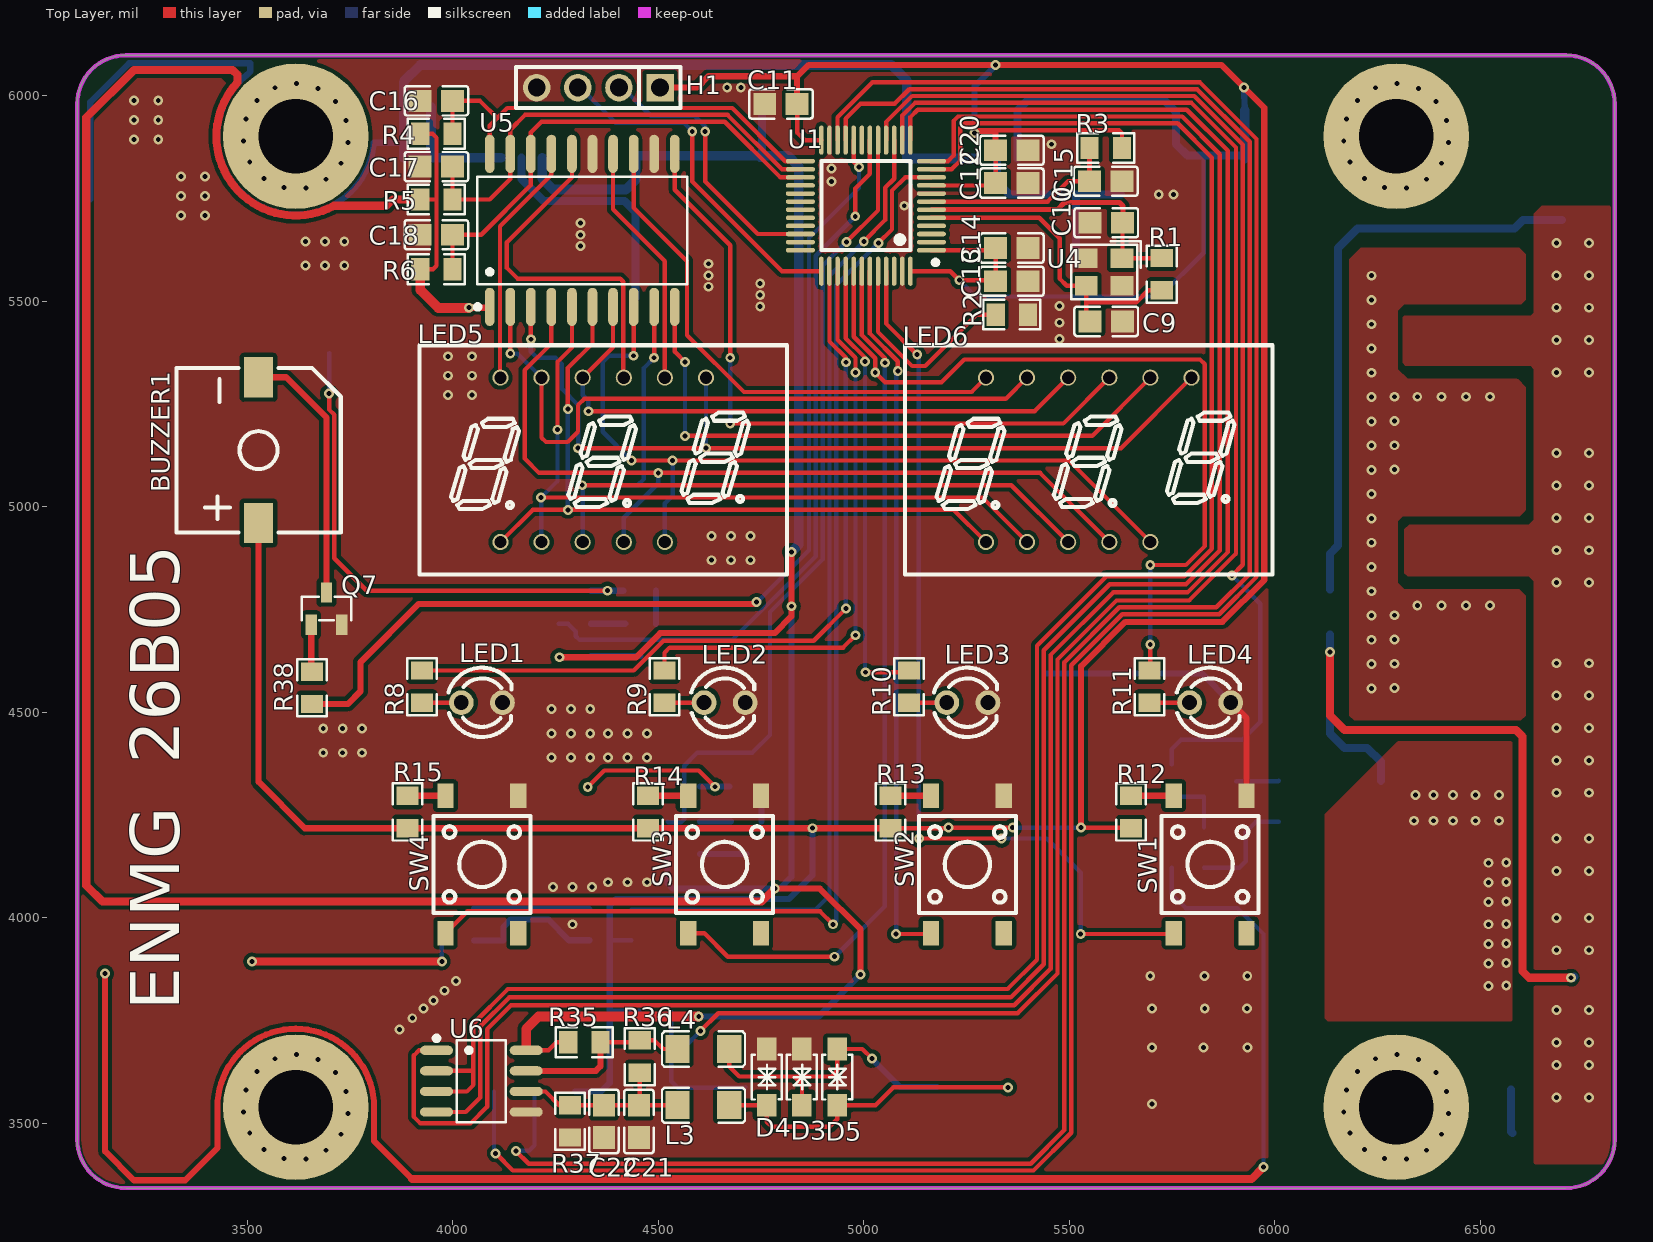
[diagram p0: Top Layer view]
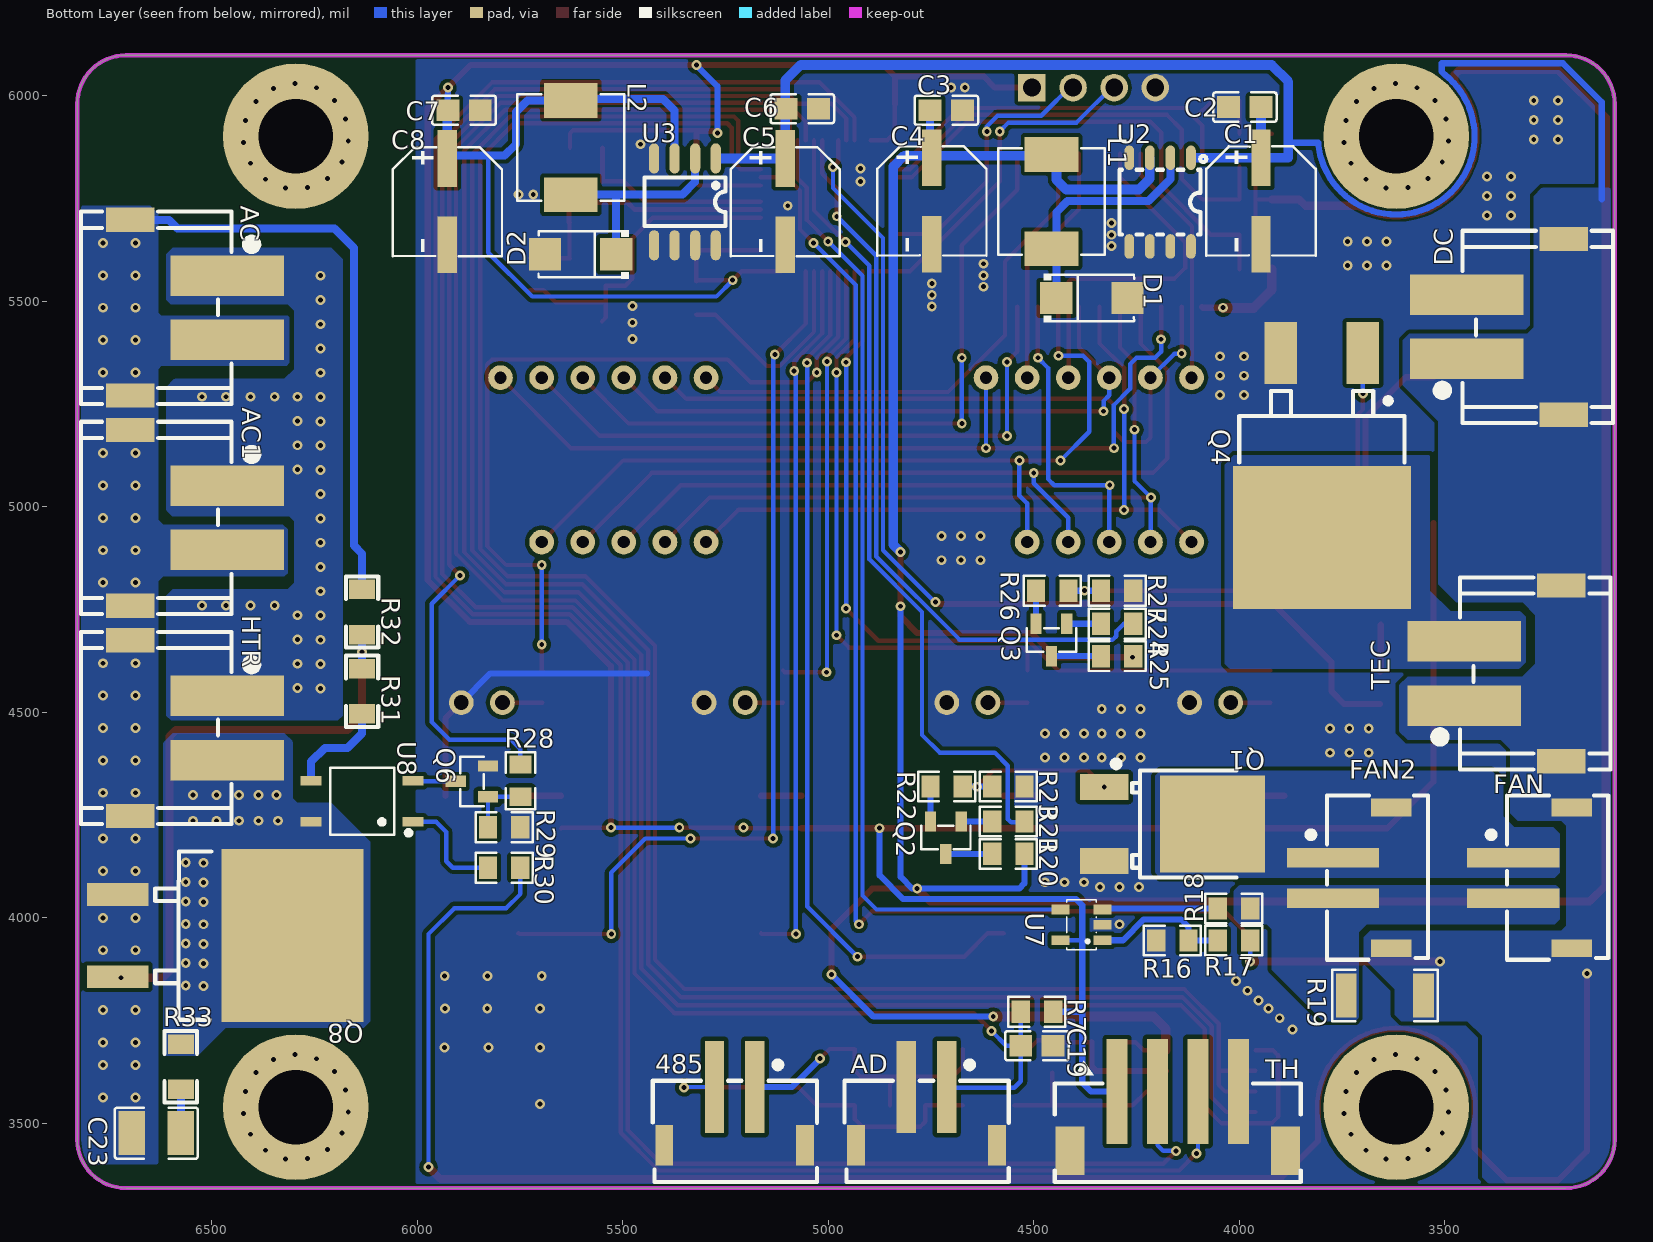
[diagram p1: Bottom Layer view, seen from below]
# Altium PCB MISC82750.pcbdoc (part 1 of 3)
Units mil, origin at the board's own origin, x right, y up, seen from the top; angles counter-clockwise.
Board outline 3740.2 x 2755.9 mil, 2 copper layers (Top Layer, Bottom Layer), stack 62.2 mil thick; 106 components, 84 nets, 362 pads, 334 vias.

## Layer stack, top to bottom
Top Solder Mask Layer: solder mask 0.4, Dk 3.3
Top Layer: signal copper 1.4
Dielectric1: surface 59.4, FR4, Dk 4.5
Bottom Layer: signal copper 1.4
Bottom Solder Mask Layer: solder mask 0.4, Dk 3.3

## Board outline
3204.7,6098.4 ccw(c3204.7,5980.3) 3086.6,5980.3 3086.6,3460.6 ccw(c3204.7,3460.6) 3204.7,3342.5 6708.7,3342.5 ccw(c6708.7,3460.6) 6826.8,3460.6 6826.8,5980.3 ccw(c6708.7,5980.3) 6708.7,6098.4

## Design rules (kind name [scope] priority, off if disabled: settings)
BoardOutlineClearance copperThickness1oz [All] p0: genericclearance=10 ignorepadtopadclearanceinfootprint=FALSE except(0: Arc-SplitContinuation Track-SplitContinuation SMDPad-SplitContinuation THPad-SplitContinuation Via-SplitContinuation Fill-SplitContinuation Poly-SplitContinuation Region-SplitContinuation Text-SplitContinuation)
BoardOutlineClearance copperThickness2oz [All] p0: genericclearance=10 ignorepadtopadclearanceinfootprint=FALSE except(0: Arc-SplitContinuation Track-SplitContinuation SMDPad-SplitContinuation THPad-SplitContinuation Via-SplitContinuation Fill-SplitContinuation Poly-SplitContinuation Region-SplitContinuation Text-SplitContinuation)
BoardOutlineClearance Plane_innerPlane [All] p0: genericclearance=10 ignorepadtopadclearanceinfootprint=FALSE except(0: Arc-SplitContinuation Track-SplitContinuation SMDPad-SplitContinuation THPad-SplitContinuation Via-SplitContinuation Fill-SplitContinuation Poly-SplitContinuation Region-SplitContinuation Text-SplitContinuation)
BoardOutlineClearance Copper_copperRegion [All] p0: genericclearance=10 ignorepadtopadclearanceinfootprint=FALSE except(0: Arc-SplitContinuation Track-SplitContinuation SMDPad-SplitContinuation THPad-SplitContinuation Via-SplitContinuation Fill-SplitContinuation Poly-SplitContinuation Region-SplitContinuation Text-SplitContinuation)
BoardOutlineClearance otherClearance [All] p0: genericclearance=10 ignorepadtopadclearanceinfootprint=FALSE except(0: Arc-SplitContinuation Track-SplitContinuation SMDPad-SplitContinuation THPad-SplitContinuation Via-SplitContinuation Fill-SplitContinuation Poly-SplitContinuation Region-SplitContinuation Text-SplitContinuation)
Clearance copperThickness1oz [All] p1: gap=7 ignorepadtopadclearanceinfootprint=FALSE
Clearance copperThickness2oz [All] p1: gap=7 ignorepadtopadclearanceinfootprint=FALSE
Clearance Plane_innerPlane [All] p1: gap=7 ignorepadtopadclearanceinfootprint=FALSE
Clearance Copper_copperRegion [All] p1: gap=7 ignorepadtopadclearanceinfootprint=FALSE
Clearance otherClearance [All] p1: gap=7 ignorepadtopadclearanceinfootprint=FALSE
DiffPairsRouting differentialPair [All] p1: maxuncoupledlength=10 minlimit=6 maxlimit=Infinity mostfreqgap=6 toplayer_minwidth=5 toplayer_prefwidth=10 toplayer_maxwidth=100 bottomlayer_minwidth=5 bottomlayer_prefwidth=10 bottomlayer_maxwidth=100
PasteMaskExpansion pasteMaskExpansion [All] p1: expansion=0
PlaneConnect innerPlane [All] p1: planeconnectstyle=Relief reliefexpansion=20 reliefentries=4 reliefconductorwidth=10 reliefairgap=10
PolygonConnect copperRegion [All] p1: connectstyle=Direct reliefentries=4 reliefconductorwidth=10 polygonreliefangle="90 Angle" airgapwidth=10
RoutingVias viaSize [All] p1: viastyle="Through Hole" holewidth=12.0078 minholewidth=11.811 maxholewidth=248.0314 width=12.0078 minwidth=11.811 maxwidth=248.0314
SolderMaskExpansion solderMaskExpansion [IsVia] p1: useseparateexpansions=TRUE expansion=-1000 expansionbottom=-1000
SolderMaskExpansion solderMaskExpansion [All] p2: useseparateexpansions=TRUE expansion=2 expansionbottom=2
Width copperThickness1oz [All] p1: maxlimit=100 minlimit=5 preferedwidth=10
Width copperThickness2oz [All] p1: maxlimit=100 minlimit=8 preferedwidth=10
Width trackWidth1 [All] p1: maxlimit=100 minlimit=5 preferedwidth=30

## Components (designator, comment, footprint, x,y, rotation, side; value= is the part's Value field where it differs from the comment)
485 "XH2.54-2P立贴" CONN-SMD_2P_A2501WV-S#1 5227.5,3517.5 r180 bottom
AC "VH3.96-2P 立贴" CONN-SMD_2P-P3.96_HCTL_HC-VH-2ALT#1 6580,5484.3 r270 bottom
AC1 "VH3.96-2P 立贴" CONN-SMD_2P-P3.96_HCTL_HC-VH-2ALT#2 6580,4973 r270 bottom
AD "XH2.54-2P立贴" CONN-SMD_2P_A2501WV-S#2 4760.9,3517.5 r180 bottom
BUZZER1 "2.7kHz" BUZ-SMD_L9.6-W9.6-LS10.0-R 3527.6,5137.8 r270 top
C1 "220uF" CAP-SMD_BD6.3-L6.6-W6.6-FD#1 3947.2,5744 r270 bottom
C2 "100nF" C0805#1 3986.5,5972.4 r0 bottom
C3 "100nF" C0805#2 4712.6,5964.6 r0 bottom
C4 "220uF" CAP-SMD_BD6.3-L6.6-W6.6-FD#1 4747.8,5744 r270 bottom
C5 "220uF" CAP-SMD_BD6.3-L6.6-W6.6-FD#2 5104.6,5742.2 r270 bottom
C6 "100nF" C0805#2 5063,5968.5 r180 bottom
C7 "100nF" C0805#1 5885.8,5964.6 r0 bottom
C8 "220uF" CAP-SMD_BD6.3-L6.6-W6.6-FD#2 5926.6,5742.2 r270 bottom
C9 "20pF" C0805#2 5589.8,5451 r180 top
C10 "20pF" C0805#2 5589.8,5691 r0 top
C11 "100nF" C0805#1 4798.3,5980 r0 top
C12 "100nF" C0805#3 5360,5787.5 r180 top
C13 "100nF" C0805#3 5360,5548.7 r180 top
C14 "100nF" C0805#3 5360,5629.4 r180 top
C15 "100nF" C0805#2 5588.6,5791.9 r180 top
C16 "100pF" C0805#1 3960,5987.5 r0 top
C17 "100pF" C0805#1 3960,5827.5 r0 top
C18 "100pF" C0805#1 3960,5662 r0 top
C19 "100nF" C0805#1 4492.1,3689 r0 bottom
C20 "100nF" C0805#3 5360,5867.5 r180 top
C21 "100nF" C0805#1 4452.9,3504.8 r90 top
C22 "100nF" C0805#1 4367.9,3504.8 r90 top
C23 "10nF" C1210 6634.5,3476.4 r180 bottom
D1 "SS34" SMA_L4.3-W2.6-LS5.2-RD 4358.3,5507.9 r180 bottom
D2 "SS34" SMA_L4.3-W2.6-LS5.2-RD 5602.4,5614.2 r0 bottom
D3 "SMF36CA" SOD-123_L2.7-W1.8-LS3.7-BI 4849.5,3612.5 r90 top
D4 "SMF36CA" SOD-123_L2.7-W1.8-LS3.7-BI 4763.9,3612.5 r90 top
D5 "SMF36CA" SOD-123_L2.7-W1.8-LS3.7-BI 4935,3612.5 r90 top
DC "VH3.96-2P 立贴" CONN-SMD_2P-P3.96_HCTL_HC-VH-2ALT#3 3328.7,5437.5 r90 bottom
FAN "XH2.54-2P立贴" CONN-SMD_2P_A2501WV-S#3 3262.4,4097.2 r90 bottom
FAN2 "XH2.54-2P立贴" CONN-SMD_2P_A2501WV-S#4 3700.8,4097.2 r90 bottom
H1 "PZ254V-11-04P" HDR-TH_4P-P2.54-V-M 4354.3,6019.7 r180 top
HTR "VH3.96-2P 立贴" CONN-SMD_2P-P3.96_HCTL_HC-VH-2ALT#2 6580,4461.8 r270 bottom
L1 "68uH" IND-SMD_L7.1-W6.6_H5.0 4456.7,5742.6 r270 bottom
L2 "68uH" IND-SMD_L7.1-W6.6_H5.0 5626,5874 r270 bottom
L3 "22uH" L1206 4610,3544.2 r0 top
L4 "22uH" L1206 4610,3680.8 r0 top
LED1 "3mmFIR" LED-TH_BD3.0-P2.54-FD 4070.9,4523.6 r0 top
LED2 "3mmFIR" LED-TH_BD3.0-P2.54-FD 4661.4,4523.6 r0 top
LED3 "3mmFIR" LED-TH_BD3.0-P2.54-FD 5252,4523.6 r0 top
LED4 "3mmFIR" LED-TH_BD3.0-P2.54-FD 5842.5,4523.6 r0 top
LED5 "SP420361N" LED-SEG-TH_SP420361N 4366.1,5114.2 r270 top
LED6 "SP420361N" LED-SEG-TH_SP420361N 5547.2,5114.2 r270 top
Q1 "NCE0140K2-VB" TO-252-3_L6.6-W6.1-P4.58-LS10.1-BR 4196.9,4228.3 r0 bottom
Q2 "SS8050(RANGE:200-350)" SOT-23-3_L2.9-W1.3-P1.90-LS2.4-BR#1 4713.9,4195 r90 bottom
Q3 "SS8050(RANGE:200-350)" SOT-23-3_L2.9-W1.3-P1.90-LS2.4-BR#2 4456.9,4675.9 r90 bottom
Q4 "HYG025N06LS1B" TO-263-2_L10.2-W8.7-P5.08-LS15.1-BR 3799.2,5149.6 r90 bottom
Q6 "SS8050(RANGE:200-350)" SOT-23-3_L2.9-W1.3-P1.90-LS2.4-BR#2 5867,4331.9 r180 bottom
Q7 "SS8050(RANGE:200-350)" SOT-23-3_L2.9-W1.3-P1.90-LS2.4-BR#1 3693,4752.4 r270 top
Q8 "BTA216B-600D-JSM" TO-263-3_L10.2-W9.2-P5.08-LS15.4-BR 6515.7,3956.7 r0 bottom
R1 "1MΩ" R0805#1 5724.8,5566 r270 top
R2 "10kΩ" R0805#1 5360,5467.5 r180 top
R3 "10kΩ" R0805#2 5588.6,5873.1 r0 top
R4 "10kΩ" R0805#1 3960,5907.5 r180 top
R5 "10kΩ" R0805#1 3960,5747.5 r180 top
R6 "10kΩ" R0805#1 3960,5578.1 r180 top
R7 "10kΩ" R0805#1 4492.1,3771.7 r180 bottom
R8 "100Ω" R0805#2 3925,4562.5 r90 top
R9 "100Ω" R0805#2 4515,4562.5 r90 top
R10 "100Ω" R0805#2 5110,4562.5 r90 top
R11 "100Ω" R0805#2 5695,4562.5 r90 top
R12 "4.7kΩ" R0805#2 5650,4257.5 r270 top
R13 "4.7kΩ" R0805#2 5065,4257.5 r270 top
R14 "4.7kΩ" R0805#2 4475,4257.5 r270 top
R15 "4.7kΩ" R0805#2 3890,4257.5 r270 top
R16 "24kΩ" R0805#1 4163,3944.9 r0 bottom
R17 "1kΩ" R0805#3 4013,3944.9 r180 bottom
R18 "1kΩ" R0805#3 4013,4022.7 r180 bottom
R19 "10mΩ" R2010 3645.7,3811 r180 bottom
R20 "4.7kΩ" R0805#3 4561.9,4155.6 r0 bottom
R21 "1kΩ" R0805#3 4561.9,4234.4 r0 bottom
R22 "10K" R0805#1 4711.9,4319.4 r180 bottom
R23 "10kΩ" R0805#3 4561.9,4319.4 r0 bottom
R24 "1kΩ" R0805#3 4296.9,4715.3 r0 bottom
R25 "4.7kΩ" R0805#3 4296.9,4636.6 r0 bottom
R26 "10K" R0805#3 4455,4795.9 r180 bottom
R27 "10kΩ" R0805#3 4296.9,4795.9 r0 bottom
R28 "10K" R0805#1 5748.8,4333.8 r270 bottom
R29 "10K" R0805#2 5788.2,4220.5 r180 bottom
R30 "10K" R0805#2 5788.2,4122 r180 bottom
R31 "51Ω" R0204 6133.9,4551.2 r90 bottom
R32 "150Ω" R0204 6133.9,4744.1 r90 bottom
R33 "120Ω" R0204 6574.8,3637.8 r90 bottom
R35 "47kΩ" R0805#1 4320,3697.5 r180 top
R36 "12kΩ" R0805#2 4455,3662.5 r90 top
R37 "47kΩ" R0805#3 4285,3504.8 r90 top
R38 "1kΩ" R0805#1 3657.5,4559.5 r90 top
SW1 "1TS005F-2500-5001" SW-SMD_4P-L6.0-W6.0-P4.50-LS9.0-H2.5#1 5842.5,4129.9 r90 top
SW2 "1TS005F-2500-5001" SW-SMD_4P-L6.0-W6.0-P4.50-LS9.0-H2.5#2 5252,4129.9 r90 top
SW3 "1TS005F-2500-5001" SW-SMD_4P-L6.0-W6.0-P4.50-LS9.0-H2.5#1 4661.4,4129.9 r90 top
SW4 "1TS005F-2500-5001" SW-SMD_4P-L6.0-W6.0-P4.50-LS9.0-H2.5#2 4070.9,4129.9 r90 top
TEC "VH3.96-2P 立贴" CONN-SMD_2P-P3.96_HCTL_HC-VH-2ALT#4 3334.6,4594.5 r90 bottom
TH "HX 2.54-4P LT" CONN-SMD_4P-P2.50_HX-2.54-4P-LT 4149.6,3505.7 r180 bottom
U1 "GD32F103C8T6" TQFP-48_L7.0-W7.0-P0.50-LS9.0-BL 5005,5732.5 r90 top
U2 "XL1509-5.0" SOIC-8_L4.9-W3.9-P1.27-LS6.0-TR 4192.6,5741.2 r180 bottom
U3 "XL1509-3.3E1" SOP-8_L4.9-W3.9-P1.27-LS6.0-BL 5348.6,5741.8 r0 bottom
U4 "8MHz" CRYSTAL-SMD_4P-L3.2-W2.5-BL 5584.8,5571 r180 top
U5 "TM1620" SOIC-20_L13.0-W7.6-P1.27-LS10.3-BL 4315,5672.5 r0 top
U6 "MAX485ESA(UMW)" SOP-8_L5.0-W4.0-P1.27-LS6.0-BL 4069.6,3602.7 r270 top
U7 "LMV321" SOT-23-5_L3.0-W1.7-P0.95-LS2.8-BR 4383.7,3983 r180 bottom
U8 "ELM3083(TA)-V" SOP-4_L4.4-W4.0-P2.54-LS7.0-TL 6133.9,4283.5 r0 bottom

## Footprints (in the part's own frame and the unit in brackets; to place one, negate y for a bottom-side part, rotate by r counter-clockwise, add the part's x,y. Pads: shape width x height; smd on the part's side, far side on the other; paste and mask are expansions set on the pad)
BUZ-SMD_L9.6-W9.6-LS10.0-R [mil]
  rect 98.4x70.9 smd: 1(177.2,0) 2(-177.2,0)
  silkscreen extent -200,-200 200,200
C0805#1 [mil]
  rect 55.5x53.1 smd paste-3937 mask+2: 1(-39.3,0) 2(39.4,0)
  silkscreen extent -77,-36 77,36
C0805#2 [mil]
  rect 55.5x53.1 smd paste-3937 mask+2: 1(-39.4,0) 2(39.4,0)
  silkscreen extent -77,-36 77,36
C0805#3 [mil]
  rect 55.5x53.1 smd paste-3937 mask+2: 1(-39.4,0) 2(39.3,0)
  silkscreen extent -77,-36 77,36
C1210 [mil]
  rect 64.4x106.3 smd paste-3937 mask+2: 1(-59.8,0) 2(59.7,0)
  silkscreen extent -101,-62 101,62
CAP-SMD_BD6.3-L6.6-W6.6-FD#1 [mil]
  rect 137.8x47.2 smd: 1(-105.1,0) 2(105.1,0)
  silkscreen extent -133,-133 133,133
CAP-SMD_BD6.3-L6.6-W6.6-FD#2 [mil]
  rect 137.8x47.2 smd: 1(-105.2,0) 2(105.1,0)
  silkscreen extent -133,-133 133,133
CONN-SMD_2P-P3.96_HCTL_HC-VH-2ALT#1 [mil]
  rect 98.4x275.6 smd paste+0 mask+2: 1(-77.9,118.1) 2(78,118.1)
  rect 59.1x118.1 smd paste+0 mask+2: 3(213.8,-118.1) 4(-213.7,-118.1)
  silkscreen extent -234,-238 234,189
CONN-SMD_2P-P3.96_HCTL_HC-VH-2ALT#2 [mil]
  rect 98.4x275.6 smd paste+0 mask+2: 1(-78,118.1) 2(77.9,118.1)
  rect 59.1x118.1 smd paste+0 mask+2: 3(213.8,-118.1) 4(-213.8,-118.1)
  silkscreen extent -234,-238 234,189
CONN-SMD_2P-P3.96_HCTL_HC-VH-2ALT#3 [mil]
  rect 98.4x275.6 smd paste+0 mask+2: 1(-77.9,118.2) 2(78,118.2)
  rect 59.1x118.1 smd paste+0 mask+2: 3(213.8,-118.1) 4(-213.8,-118.1)
  silkscreen extent -234,-238 234,189
CONN-SMD_2P-P3.96_HCTL_HC-VH-2ALT#4 [mil]
  rect 98.4x275.6 smd paste+0 mask+2: 1(-78,118.2) 2(77.9,118.2)
  rect 59.1x118.1 smd paste+0 mask+2: 3(213.8,-118.1) 4(-213.8,-118.1)
  silkscreen extent -234,-238 234,189
CONN-SMD_2P_A2501WV-S#1 [mil]
  rect 47.2x224.4 smd paste+0 mask+2: 1(49.2,70.9) 2(-49.2,70.9)
  rect 43.3x98.4 smd paste+0 mask+2: 3(-171.3,-70.8) 4(171.2,-70.8)
  silkscreen extent -199,-160 200,133
CONN-SMD_2P_A2501WV-S#2 [mil]
  rect 47.2x224.4 smd paste+0 mask+2: 1(49.2,70.9) 2(-49.3,70.9)
  rect 43.3x98.4 smd paste+0 mask+2: 3(-171.3,-70.8) 4(171.2,-70.8)
  silkscreen extent -199,-160 200,133
CONN-SMD_2P_A2501WV-S#3 [mil]
  rect 47.2x224.4 smd paste+0 mask+2: 1(49.2,70.8) 2(-49.3,70.8)
  rect 43.3x98.4 smd paste+0 mask+2: 3(-171.3,-70.9) 4(171.2,-70.9)
  silkscreen extent -199,-160 200,133
CONN-SMD_2P_A2501WV-S#4 [mil]
  rect 47.2x224.4 smd paste+0 mask+2: 1(49.2,70.9) 2(-49.3,70.9)
  rect 43.3x98.4 smd paste+0 mask+2: 3(-171.3,-70.9) 4(171.2,-70.9)
  silkscreen extent -199,-160 200,133
CONN-SMD_4P-P2.50_HX-2.54-4P-LT [mil]
  rect 51.2x255.9 smd paste+0 mask+2: 1(-147.6,71.9) 2(-49.2,71.9) 3(49.2,71.9) 4(147.6,71.9)
  rect 70.9x118.1 smd paste+0 mask+2: 5(261.8,-71.8) 6(-261.8,-71.8)
  silkscreen extent -299,-149 299,147
CRYSTAL-SMD_4P-L3.2-W2.5-BL [mil]
  rect 55.1x47.2 smd: 1(-43.3,-33.5) 2(43.3,-33.5) 3(43.3,33.4) 4(-43.3,33.4)
  silkscreen extent -89,-75 80,66
HDR-TH_4P-P2.54-V-M [mil]
  rect 66.9x66.9 hole 43.3: 1(-150,0)
  round 66.9 hole 43.3: 2(-50,0) 3(50,0) 4(150,0)
  silkscreen extent -200,-50 200,50
IND-SMD_L7.1-W6.6_H5.0 [mil]
  rect 84.6x130.7 smd: 1(-114.7,0) 2(114.7,0)
  silkscreen extent -130,-130 130,130
L1206 [mil]
  rect 58.5x68 smd paste-3937 mask+2: 1(-62.7,0) 2(62.7,0)
  silkscreen extent -101,-43 101,43
LED-SEG-TH_SP420361N [mil]
  round 39.4 / inner round 39.4 / far side round 60 hole 30: 1(200,-250) 2(200,-150) 3(200,-50) 4(200,50) 5(200,150) 7(-200,250) 8(-200,150) 9(-200,50) 10(-200,-50) 11(-200,-150) 12(-200,-250)
  silkscreen extent -279,-447 279,447
LED-TH_BD3.0-P2.54-FD [mil]
  round 60 hole 36: 1(-50,0) 2(50,0)
  silkscreen extent -81,-84 72,85
R0204 [mil]
  rect 47.2x63 smd paste+0 mask+2: 1(-55.1,0) 2(55.1,0)
  silkscreen extent -87,-39 87,39
R0805#1 [mil]
  rect 44.6x54.2 smd paste-3937 mask+2: 1(-39.4,0) 2(39.3,0)
  silkscreen extent -69,-36 69,36
R0805#2 [mil]
  rect 44.6x54.2 smd paste-3937 mask+2: 1(-39.4,0) 2(39.4,0)
  silkscreen extent -69,-36 69,36
R0805#3 [mil]
  rect 44.6x54.2 smd paste-3937 mask+2: 1(-39.3,0) 2(39.4,0)
  silkscreen extent -69,-36 69,36
R2010 [mil]
  rect 50.5x106.3 smd paste-3937 mask+2: 1(-94.1,0) 2(94.2,0)
  silkscreen extent -128,-62 128,62
SMA_L4.3-W2.6-LS5.2-RD [mil]
  rect 78.7x78.7 smd: 1(-86.6,0) 2(86.6,0)
  silkscreen extent -117,-59 102,59
SOD-123_L2.7-W1.8-LS3.7-BI [mil]
  rect 55.1x47.2 smd: 1(-68.3,0) 2(68.3,0)
  silkscreen extent -54,-36 54,36
SOIC-8_L4.9-W3.9-P1.27-LS6.0-TR [mil]
  oval 23.6x59.8 smd: 1(75,107.9) 2(25,107.9) 3(-25,107.9) 4(-75,107.9) 5(-75,-107.8) 6(-25,-107.8) 7(25,-107.8) 8(75,-107.8)
  silkscreen extent -98,-79 113,112
SOIC-20_L13.0-W7.6-P1.27-LS10.3-BL [mil]
  oval 23.4x92.9 smd: 1(-225,-186.2) 2(-175,-186.2) 3(-125,-186.2) 4(-75,-186.2) 5(-25,-186.2) 6(25,-186.2) 7(75,-186.2) 8(125,-186.2) 9(175,-186.2) 10(225,-186.2) 11(225,186.2) 12(175,186.2) 13(125,186.2) 14(75,186.2) 15(25,186.2) 16(-25,186.2) 17(-75,186.2) 18(-125,186.2) 19(-175,186.2) 20(-225,186.2)
  silkscreen extent -260,-192 255,131
SOP-4_L4.4-W4.0-P2.54-LS7.0-TL [mil]
  rect 51.2x23.4 smd: 1(-124.1,50) 2(-124.1,-50) 3(124,-50) 4(124,50)
  silkscreen extent -119,-82 78,82
SOP-8_L4.9-W3.9-P1.27-LS6.0-BL [mil]
  oval 24.8x73.4 smd: 1(-75,-105.6) 2(-25,-105.6) 3(25,-105.6) 4(75,-105.6) 5(75,105.7) 6(25,105.7) 7(-25,105.7) 8(-75,105.7)
  silkscreen extent -98,-59 98,58
SOP-8_L5.0-W4.0-P1.27-LS6.0-BL [mil]
  oval 22.6x80.1 smd: 1(-75,-109) 2(-25,-109) 3(25,-109) 4(75,-109) 5(75,109) 6(25,109) 7(-25,109) 8(-75,109)
  silkscreen extent -110,-115 100,60
SOT-23-3_L2.9-W1.3-P1.90-LS2.4-BR#1 [mil]
  rect 49.2x27.6 smd: 1(39.4,-37.4) 2(39.4,37.4) 3(-39.4,0)
  silkscreen extent -29,-60 29,60
SOT-23-3_L2.9-W1.3-P1.90-LS2.4-BR#2 [mil]
  rect 49.2x27.6 smd: 1(39.4,-37.4) 2(39.4,37.4) 3(-39.3,0)
  silkscreen extent -29,-60 29,60
SOT-23-5_L3.0-W1.7-P0.95-LS2.8-BR [mil]
  rect 43.3x23.6 smd: 1(51.1,-37.4) 2(51.1,0) 3(51.1,37.4) 4(-51.2,37.4) 5(-51.2,-37.4)
  silkscreen extent -36,-61 35,61
SW-SMD_4P-L6.0-W6.0-P4.50-LS9.0-H2.5#1 [mil]
  rect 59.1x39.4 smd: 1(-167.3,88.6) 2(167.3,88.6) 3(-167.3,-88.6) 4(167.3,-88.6)
  silkscreen extent -118,-118 118,118
SW-SMD_4P-L6.0-W6.0-P4.50-LS9.0-H2.5#2 [mil]
  rect 59.1x39.4 smd: 1(-167.3,88.6) 2(167.3,88.6) 3(-167.3,-88.5) 4(167.3,-88.5)
  silkscreen extent -118,-118 118,118
TO-252-3_L6.6-W6.1-P4.58-LS10.1-BR [mil]
  rect 118.1x63 smd: 1(131.5,-90) 2(131.5,89.9)
  rect 255.9x236.2 smd: 3(-131.6,0)
  silkscreen extent -190,-154 110,130
TO-263-2_L10.2-W8.7-P5.08-LS15.1-BR [mil]
  rect 150x78.7 smd: 1(224.5,-100) 3(224.6,100)
  rect 348x433.1 smd: 4(-224.5,0)
  silkscreen extent -41,-201 132,201
TO-263-3_L10.2-W9.2-P5.08-LS15.4-BR [mil]
  rect 149.6x55.1 smd: 1(212.6,-100) 3(212.6,100)
  rect 346.5x421.3 smd: 2(-212.5,0)
  silkscreen extent -15,-205 121,205
TQFP-48_L7.0-W7.0-P0.50-LS9.0-BL [mil]
  oval 11x70.9 smd: 1(-108.3,-159.5) 2(-88.6,-159.5) 3(-68.9,-159.5) 4(-49.2,-159.5) 5(-29.5,-159.5) 6(-9.8,-159.5) 7(9.9,-159.5) 8(29.5,-159.5) 9(49.2,-159.5) 10(68.9,-159.5) 11(88.6,-159.5) 12(108.3,-159.5) 25(108.3,159.4) 26(88.6,159.4) 27(68.9,159.4) 28(49.2,159.4) 29(29.5,159.4) 30(9.9,159.4) 31(-9.8,159.4) 32(-29.5,159.4) 33(-49.2,159.4) 34(-68.9,159.4) 35(-88.6,159.4) 36(-108.3,159.4)
  oval 70.9x11 smd: 13(159.5,-108.3) 14(159.5,-88.6) 15(159.5,-68.9) 16(159.5,-49.2) 17(159.5,-29.6) 18(159.5,-9.9) 19(159.5,9.8) 20(159.5,29.5) 21(159.5,49.2) 22(159.5,68.9) 23(159.5,88.5) 24(159.5,108.2) 37(-159.4,108.2) 38(-159.4,88.5) 39(-159.4,68.9) 40(-159.4,49.2) 41(-159.4,29.5) 42(-159.4,9.8) 43(-159.4,-9.9) 44(-159.4,-29.6) 45(-159.4,-49.2) 46(-159.4,-68.9) 47(-159.4,-88.6) 48(-159.4,-108.3)
  silkscreen extent -144,-175 108,108

## Free pads (board coordinates)
  round 354.3 / inner round 196.9 / far side round 354.3 hole 181.1: 1(3618.1,5901.6) 2(6295.3,5901.6) 3(6295.3,3539.4) 4(3618.1,3539.4)

## Via types
v1: diameter 24, hole 12, Top Layer to Bottom Layer, 334 vias

## Nets (pads, with @x,y where several pads share a name; then routed paths per layer and width w, separated by ;. In a path a pad name is that pad's centre, name@x,y a point inside that pad or via, vN(x,y) a via of type N, cw(c..) or ccw(c..) an arc to the next point about the centre after c; other vN are vias at no path point)
1: LED5.12 U5.17 | length 596.7
  Top Layer w10.6: LED5.12@4116.1,5314.2 4115,5315.3 4115,5682.5 4240,5807.5 U5.17@4240,5858.7
2: LED5.9 U5.16 | length 874.3
  Top Layer w10.6: U5.16@4290,5858.7 4290,5801.9 4131.7,5643.5 4131.7,5580.9 4157.5,5555.1 4407.5,5555.1 4415,5547.6 4415,5315.3 LED5.9@4416.1,5314.2
3: LED5.8 U5.14 | length 596.7
  Top Layer w10.6: U5.14@4390,5858.7 4390,5723.6 4516.1,5597.5 LED5.8@4516.1,5314.2
4: LED6.12 U5.13 | length 1294.1
  Top Layer w10.6: U5.13@4440,5858.7 4440,5727.5 4570,5597.5 4570,5417.5 4708.4,5279.1 5262.2,5279.1 LED6.12@5297.2,5314.2
5: LED6.9 U5.11 | length 1680.6
  Top Layer w10.6: U5.11@4540,5858.7 4540,5771 4675,5636 v1(4675,5362.5) ; v1(4675,5202.5) 5485.6,5202.5 LED6.9@5597.2,5314.2
  Bottom Layer w10.6: v1(4675,5202.5) v1(4675,5362.5)
6: LED6.8 U5.10 | length 1515.1
  Top Layer w10.6: U5.10@4540,5486.3 4540,5377.5 v1(4565,5352.5) ; v1(4565,5172.5) 5555.6,5172.5 LED6.8@5697.2,5314.2
  Bottom Layer w10.6: v1(4565,5172.5) v1(4565,5352.5)
$1N7461: D1.1 L1.2 U2.2 | length 571.3
  Bottom Layer w19.7: U2.2@4167.6,5849.1 4167.6,5797 4220.6,5744 4417.4,5744 4444.9,5716.5 4444.9,5627.9 D1.1@4444.9,5507.9
$1N7790: D2.1 L2.2 U3.2 | length 517.3
  Bottom Layer w19.7: U3.2@5323.6,5847.4 5323.6,5790.6 5354.8,5759.3 5515.8,5759.3 ; D2.1@5515.8,5614.2 5515.8,5759.3 ; L2.2@5626,5759.3 5515.8,5759.3
$2N1439: R15.1 SW4.2 | length 92.4
  Top Layer w15: R15.1@3890,4296.9 3981.9,4296.9 SW4.2@3982.3,4297.2
$2N1440: R14.1 SW3.2 | length 97.9
  Top Layer w15: R14.1@4475,4296.9 4572.5,4296.9 SW3.2@4572.8,4297.2
$2N1441: R13.1 SW2.2 | length 98.5
  Top Layer w15: R13.1@5065,4296.9 5163,4296.9 SW2.2@5163.4,4297.2
$2N1442: R12.1 SW1.2 | length 104
  Top Layer w15: R12.1@5650,4296.9 5753.6,4296.9 SW1.2@5753.9,4297.2
$2N2869: Q4.1 R26.2 R27.2 | length 1281.5
  Top Layer w10.6: v1(3699.2,5275.6) 3699.2,5236.8 3711.8,5224.3 3711.8,4874.8 3790.7,4795.9 v1(4376.8,4795.9)
  Bottom Layer w10.6: v1(3699.2,5275.6) Q4.1@3699.2,5374.1
  Bottom Layer w15: R27.2@4336.3,4795.9 v1(4376.8,4795.9) R26.2@4415.6,4795.9
$2N18626: Q3.1 R24.2 | length 83.2
  Bottom Layer w15: R24.2@4336.3,4715.3 Q3.1@4419.5,4715.3
$2N18627: Q3.2 R26.1 | length 80.6
  Bottom Layer w15: Q3.2@4494.3,4715.3 R26.1@4494.3,4795.9
$2N18793: Q6.1 R28.2 R29.1 | length 152.8
  Bottom Layer w10.6: R28.2@5748.8,4294.5 Q6.1@5827.6,4294.5 R29.1@5827.6,4220.5
$2N18795: Q6.3 U8.2 | length 104.2
  Bottom Layer w10.6: Q6.3@5906.3,4331.9 6008.3,4331.9 U8.2@6009.8,4333.5
$2N19026: C23.2 R33.1 | length 107.7
  Bottom Layer w19.7: R33.1@6574.8,3582.7 6574.8,3479.6 C23.2@6578.1,3476.4
$2N19158: R31.1 U8.3 | length 246.2
  Bottom Layer w19.7: R31.1@6133.9,4496.1 6133.9,4448.8 6169.3,4413.4 6224.4,4413.4 6257.9,4379.9 U8.3@6257.9,4333.5
$2N19197: Q8.3 R31.2 R32.1 | length 1431.7
  Top Layer w19.7: v1(6133.9,4647.1) 6133.9,4492.1 6169.3,4456.7 6586.6,4456.7 6602.4,4440.9 6602.4,3870.1 6618.1,3854.3 v1(6720.5,3854.3)
  Bottom Layer w19.7: R31.2@6133.9,4606.3 v1(6133.9,4647.1) R32.1@6133.9,4689 ; v1(6720.5,3854.3) 6726,3854.3 Q8.3@6728.3,3856.7
$2N19726: R30.1 U8.1 | length 269.9
  Bottom Layer w10.6: R30.1@5827.6,4122 5913.4,4122 5929.1,4137.8 5929.1,4208.7 5953.9,4233.5 U8.1@6009.8,4233.5
$2N24660: C21.2 C22.2 L3.1 R36.1 R37.2 U6.6 | length 462.4
  Top Layer w10.6: U6.6@4178.6,3577.7 4225.5,3577.7 4258.9,3544.2 R37.2@4285,3544.2 C22.2@4367.9,3544.2 C21.2@4452.9,3544.2 ; R36.1@4455,3623.1 4455,3546.3 C21.2@4452.9,3544.2 ; L3.1@4547.3,3544.2 C21.2@4452.9,3544.2
$2N24661: L4.1 R35.1 R36.2 U6.7 | length 442.5
  Top Layer w10.6: R35.1@4359.4,3697.5 4450.7,3697.5 R36.2@4455,3701.9 4491,3701.9 4512.1,3680.8 L4.1@4547.3,3680.8
  Top Layer w15: U6.7@4178.6,3627.7 4348.2,3627.7 4359.4,3638.9 R35.1@4359.4,3697.5
$2N24685: R18.1 U7.3 | length 281.2
  Bottom Layer w15: R18.1@4052.3,4022.7 4330.2,4022.7 U7.3@4332.6,4020.4
$2N24686: R16.1 R17.1 U7.1 | length 341.8
  Bottom Layer w15: R17.1@4052.3,3944.9 R16.1@4123.6,3944.9 4123.6,3977.9 4141.7,3996.1 4232.3,3996.1 4282.8,3945.6 U7.1@4332.6,3945.6
$2N24697: Q2.1 R21.2 | length 75.2
  Bottom Layer w15: R21.2@4601.3,4234.4 Q2.1@4676.5,4234.4
$2N24698: Q2.2 R22.1 | length 85
  Bottom Layer w15: Q2.2@4751.3,4234.4 R22.1@4751.3,4319.4
$2N24700: Q1.1 R22.2 R23.2 | length 413.6
  Top Layer w10.6: v1(4328.4,4318.3) 4368.4,4358.3 4598.4,4358.3 v1(4637.8,4318.9)
  Bottom Layer w15: R23.2@4601.3,4319.4 R22.2@4672.6,4319.4
$2N24704: LED1.1 R8.1 | length 96.1
  Top Layer w10.6: R8.1@3925,4523.1 4020.4,4523.1 LED1.1@4020.9,4523.6
$2N24706: LED2.1 R9.1 | length 96.6
  Top Layer w10.6: R9.1@4515,4523.1 4610.9,4523.1 LED2.1@4611.4,4523.6
$2N24708: LED3.1 R10.1 | length 92.2
  Top Layer w10.6: R10.1@5110,4523.1 5201.5,4523.1 LED3.1@5202,4523.6
$2N24710: LED4.1 R11.1 | length 97.7
  Top Layer w10.6: R11.1@5695,4523.1 5792,4523.1 LED4.1@5792.5,4523.6
$2N24715: Q3.3 R25.2 | length 120.6
  Bottom Layer w15: R25.2@4336.3,4636.6 Q3.3@4456.9,4636.6
$2N24717: Q2.3 R20.2 | length 112.6
  Bottom Layer w15: R20.2@4601.3,4155.6 Q2.3@4713.9,4155.6
$2N24723: BUZZER1.2 Q7.3 | length 630.9
  Top Layer w15: BUZZER1.2@3527.6,5315 3594.5,5315 3693,5216.5 Q7.3@3693,4791.8
$2N24729: Q7.1 R38.2 | length 115
  Top Layer w15: Q7.1@3655.6,4713 3655.6,4600.8 R38.2@3657.5,4598.8